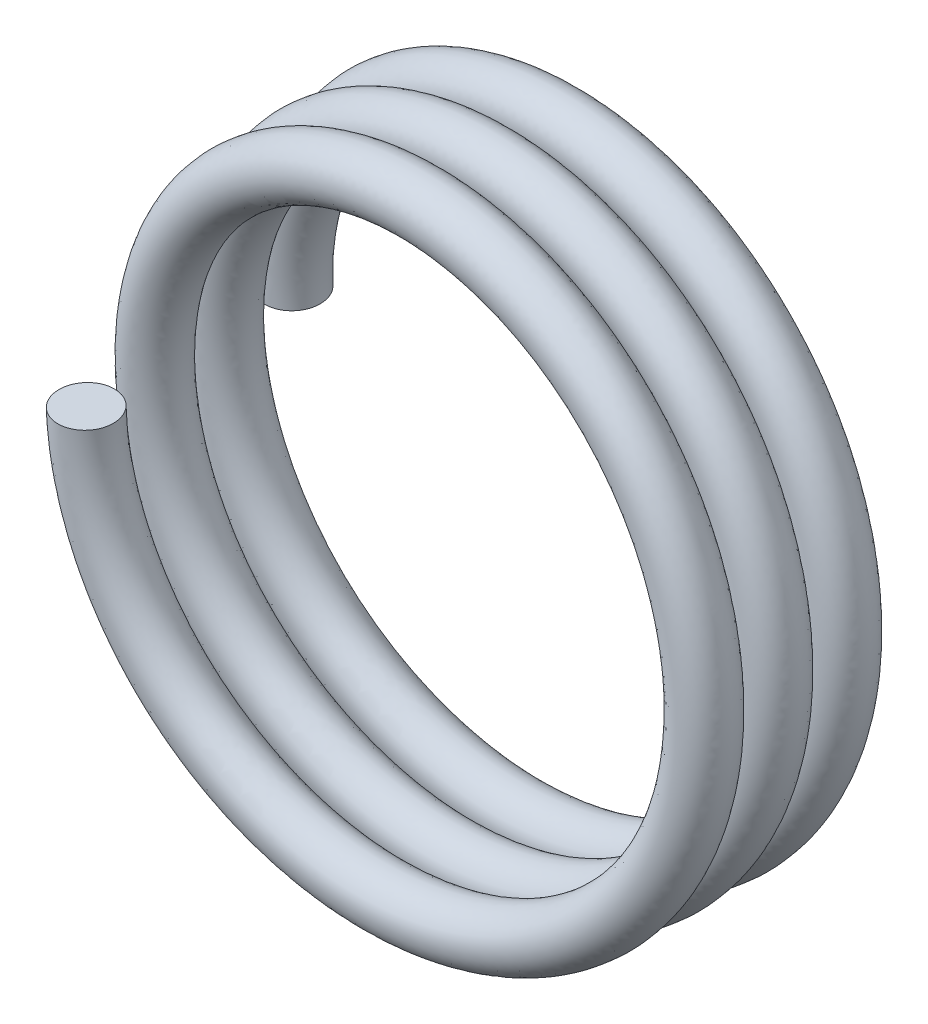
SolidWorks part; units mm, degrees
ref_plane "Front Plane" through (0, 0, 0) normal (0, 0, 1) x (1, 0, 0)
ref_plane "Top Plane" through (0, 0, 0) normal (0, 1, 0) x (1, 0, 0)
ref_plane "Right Plane" through (0, 0, 0) normal (1, 0, 0) x (0, 0, -1)
other "Configuration Table"
sketch "Sketch2" plane through (0, 0, 0) normal (0, 0, 1) x (1, 0, 0)
  circle A0 centre (0, 0) radius 7.75
  dimension "D1" = 15.5
curve "Helix/Spiral1" pitch 1.8333 height 5.5 turns 3
sweep "Sweep1" add path "Helix/Spiral1" circular profile diameter 1.5 parameters "D3"=1.5
